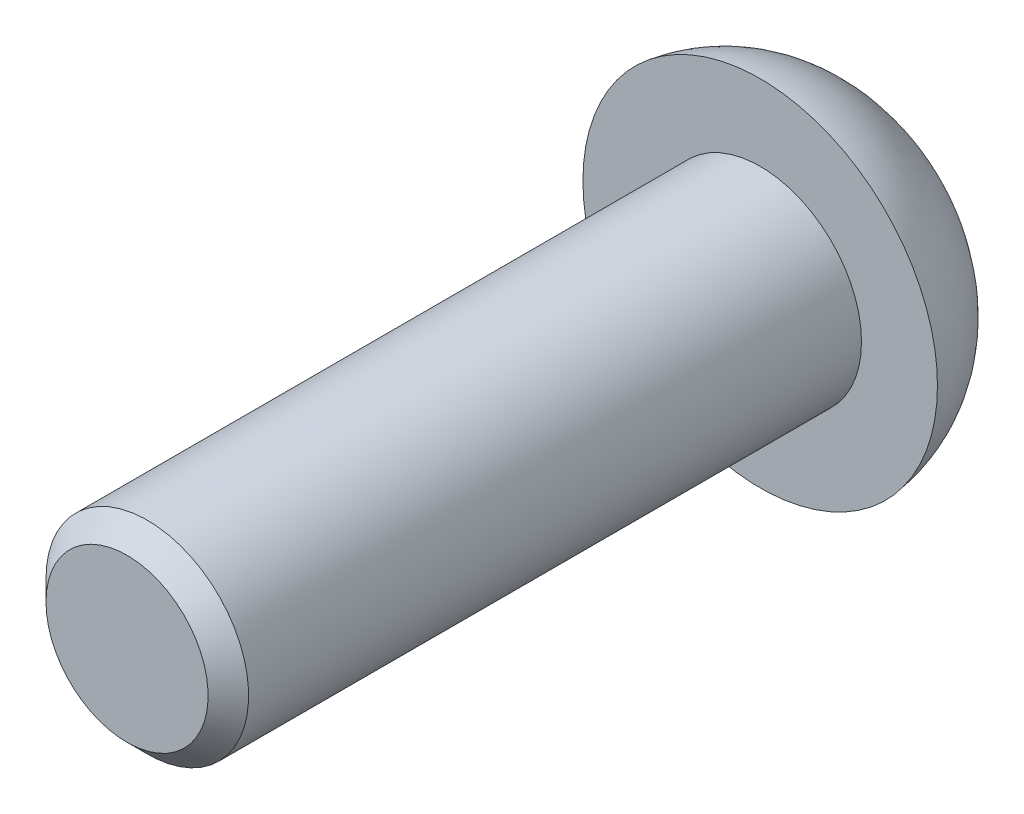
SolidWorks part; units mm, degrees
ref_plane "前视基准面" through (0, 0, 0) normal (0, 0, 1) x (1, 0, 0)
ref_plane "上视基准面" through (0, 0, 0) normal (0, 1, 0) x (1, 0, 0)
ref_plane "右视基准面" through (0, 0, 0) normal (1, 0, 0) x (0, 0, -1)
sketch "草图1" plane through (0, 0, 0) normal (0, 0, 1) x (1, 0, 0)
  circle A0 centre (0, 0) radius 7
  dimension "D1" = 14
extrude "凸台-拉伸1" add sketch "草图1" against normal blind 4.4
sketch "草图2" plane through (0, 0, 0) normal (0, 0, -1) x (-1, 0, 0)
  circle A0 centre (0, 0) radius 4
  dimension "D1" = 8
extrude "凸台-拉伸2" add sketch "草图2" against normal blind 25
cosmetic thread "装饰螺纹线1" parameters "D2"=6.647
chamfer "倒角1" distance 0.8 angle 45 1 edges at (-4, 0, 25)
sketch "草图3" plane through (0, 0, -4.4) normal (0, 0, 1) x (1, 0, 0)
  line L1 (1.4434, 2.5) -> (-1.4434, 2.5)
  line L2 (-1.4434, 2.5) -> (-2.8868, 0)
  line L3 (-2.8868, 0) -> (-1.4434, -2.5)
  line L4 (-1.4434, -2.5) -> (1.4434, -2.5)
  line L5 (1.4434, -2.5) -> (2.8868, 0)
  line L6 (2.8868, 0) -> (1.4434, 2.5)
  circle A0 centre (0, 0) radius 2.5 construction
  dimension "D1" = 5
extrude "切除-拉伸1" cut sketch "草图3" along normal blind 2.2
sketch "草图4" plane through (0, 0, 0) normal (-1, 0, 0) x (0, 1, 0)
  line L0 (0, 0) -> (0, -50000) construction
  line L1 (0, 0.7566) -> (-2.5, 2.2)
  line L2 (-2.5, 2.2) -> (0, 2.2)
  line L3 (0, 2.2) -> (0, 0.7566)
  dimension "D1" = 60
revolve "切除-旋转1" cut sketch "草图4" angle 360 about L0
sketch "草图5" plane through (0, 0, 0) normal (0, 1, 0) x (1, 0, 0)
  line L0 (-7, 0) -> (-7, 4.4)
  line L1 (-7, 4.4) -> (-3.5, 4.4)
  line L2 (7, 4.4) -> (-7, 4.4) construction
  line L3 (0, 0) -> (0, -50000) construction
  arc A0 (-3.5, 4.4) -> (-7, 0) centre (-1.6418, -0.6702) ccw
  dimension "D2" = 5.4
  dimension "D1" = 3.5
revolve "切除-旋转2" cut sketch "草图5" angle 360 about L3
